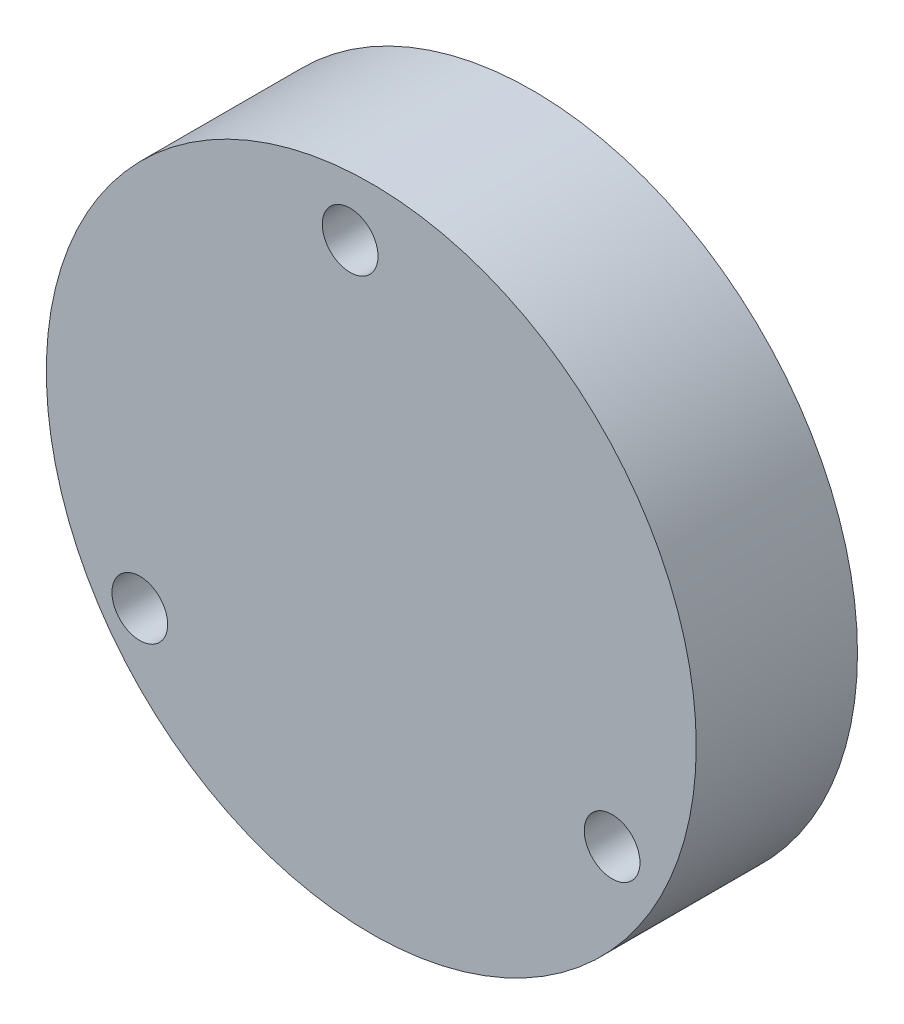
SolidWorks part; units mm, degrees
ref_plane "Front Plane" through (0, 0, 0) normal (0, 0, 1) x (1, 0, 0)
ref_plane "Top Plane" through (0, 0, 0) normal (0, 1, 0) x (1, 0, 0)
ref_plane "Right Plane" through (0, 0, 0) normal (1, 0, 0) x (0, 0, -1)
sketch "Model" plane through (0, 0, 0) normal (0, 0, 1) x (1, 0, 0)
  circle A1 centre (-16.7609, 6.7459) radius 2.5909
  circle A2 centre (-36.327, -32.6866) radius 2.5909
  circle A3 centre (7.6056, -29.9152) radius 2.5909
  circle A4 centre (-14.7956, -17.9152) radius 30.2268
  dimension "D1" = 44.02
  dimension "D2" = 44.02
  dimension "D3" = 44.02
  dimension "D4" = 12
extrude "Boss-Extrude1" add sketch "Model" along normal blind 15
